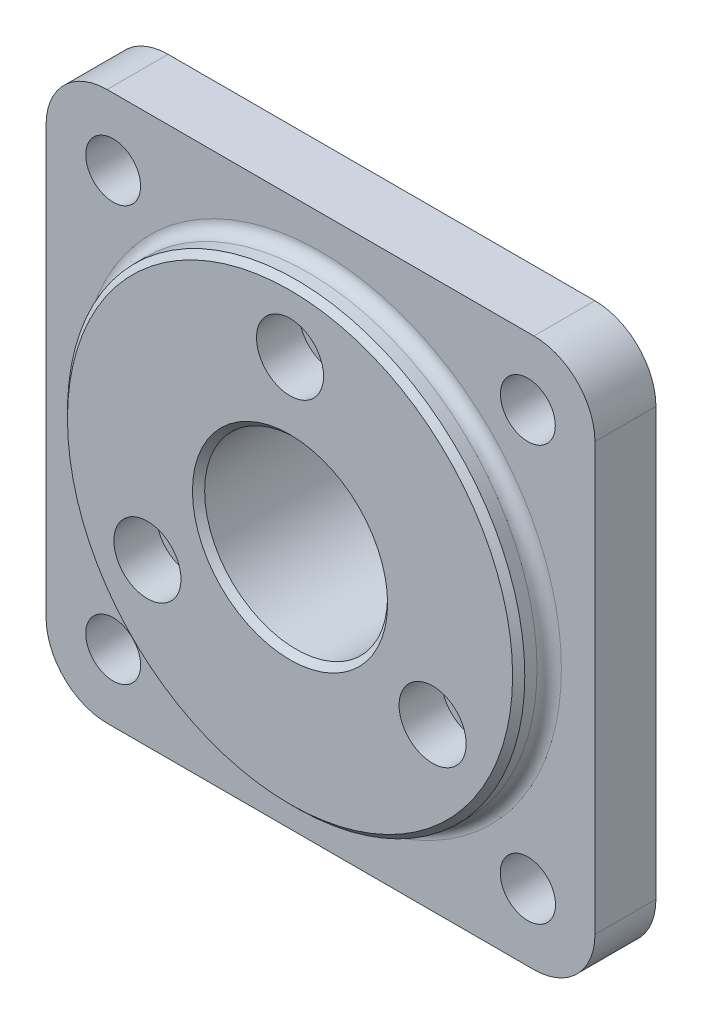
from build123d import *

# Parameters (mm, degrees)
SKETCH_1_W               = 90
SKETCH_1_H               = 90
EXTRUDE_1_DEPTH          = 10
FILLET_1_R               = 10
SKETCH_2_R               = 4.5
SKETCH_2_R_2             = 4.53
CUT_EXTRUDE_1_DEPTH      = 65.420493634
SKETCH_3_R               = 37.5
EXTRUDE_2_DEPTH          = 5
SKETCH_4_R               = 17.5
EXTRUDE_3_DEPTH          = 7
SKETCH_5_R               = 15
CUT_EXTRUDE_2_DEPTH      = 68.334983478
SKETCH_6_R               = 5.5
CUT_EXTRUDE_3_DEPTH      = 7
SKETCH_7_R               = 3.5
CUT_EXTRUDE_4_DEPTH      = 66.383484153
PATTERN_CIRCULAR_1_COUNT = 3
FILLET_2_R               = 2
CHAMFER_1_SIZE           = 1


with BuildPart() as part:
    # 草图1 → 凸台-拉伸1 (new body)
    with BuildSketch(Plane.XY):
        Rectangle(SKETCH_1_W, SKETCH_1_H)
    extrude(amount=EXTRUDE_1_DEPTH)

    # 圆角1
    fillet_1_edges = [part.edges().sort_by_distance(p)[0] for p in [
        (45, -45, 5),
        (-45, -45, 5),
        (-45, 45, 5),
        (45, 45, 5),
    ]]
    fillet(fillet_1_edges, radius=FILLET_1_R)

    # 草图2 → 切除-拉伸1 (cut, through all)
    with BuildSketch(Plane.XY.offset(10)):
        with Locations((-34, 34)):
            Circle(SKETCH_2_R)
        with Locations((34, 34)):
            Circle(SKETCH_2_R)
        with Locations((-34, -34)):
            Circle(SKETCH_2_R)
        with Locations((34, -34)):
            Circle(SKETCH_2_R_2)
    extrude(amount=-CUT_EXTRUDE_1_DEPTH, mode=Mode.SUBTRACT)

    # 草图3 → 凸台-拉伸2 (add)
    with BuildSketch(Plane.XY.offset(10)):
        Circle(SKETCH_3_R)
    extrude(amount=EXTRUDE_2_DEPTH)

    # 草图4 → 凸台-拉伸3 (add)
    with BuildSketch(Plane(origin=(0, 0, 0), x_dir=(-1, 0, 0), z_dir=(0, 0, -1))):
        with Locations(Location((0, 0, 0), (0, 0, 180))):
            Circle(SKETCH_4_R)
    extrude(amount=EXTRUDE_3_DEPTH)

    # 草图5 → 切除-拉伸2 (cut, through all)
    with BuildSketch(Plane.XY.offset(15)):
        Circle(SKETCH_5_R)
    extrude(amount=-CUT_EXTRUDE_2_DEPTH, mode=Mode.SUBTRACT)

    # 草图6 → 切除-拉伸3 (cut)
    with BuildSketch(Plane.XY.offset(15)):
        with Locations((0, 27)):
            Circle(SKETCH_6_R)
    cut_extrude_3 = extrude(amount=-CUT_EXTRUDE_3_DEPTH, mode=Mode.SUBTRACT)

    # 草图7 → 切除-拉伸4 (cut, through all)
    with BuildSketch(Plane.XY.offset(8)):
        with Locations((0, 27)):
            Circle(SKETCH_7_R)
    cut_extrude_4 = extrude(amount=-CUT_EXTRUDE_4_DEPTH, mode=Mode.SUBTRACT)

    # 阵列(圆周)1: 切除-拉伸3, 切除-拉伸4 ×3 about axis
    pattern_circular_1_axis = Axis((0, 0, 0), (0, 0, 1))
    add([cut_extrude_3.rotate(pattern_circular_1_axis, i * 360 / PATTERN_CIRCULAR_1_COUNT) for i in range(1, PATTERN_CIRCULAR_1_COUNT)], mode=Mode.SUBTRACT)
    add([cut_extrude_4.rotate(pattern_circular_1_axis, i * 360 / PATTERN_CIRCULAR_1_COUNT) for i in range(1, PATTERN_CIRCULAR_1_COUNT)], mode=Mode.SUBTRACT)

    # 圆角2
    fillet_2_edges = [part.edges().sort_by_distance(p)[0] for p in [
        (-37.5, 0, 10),
    ]]
    fillet(fillet_2_edges, radius=FILLET_2_R)

    # 倒角1
    chamfer_1_edges = [part.edges().sort_by_distance(p)[0] for p in [
        (-37.5, 0, 15),
        (-17.5, 0, -7),
        (-15, 0, 15),
    ]]
    chamfer(chamfer_1_edges, length=CHAMFER_1_SIZE)


solid = part.part
